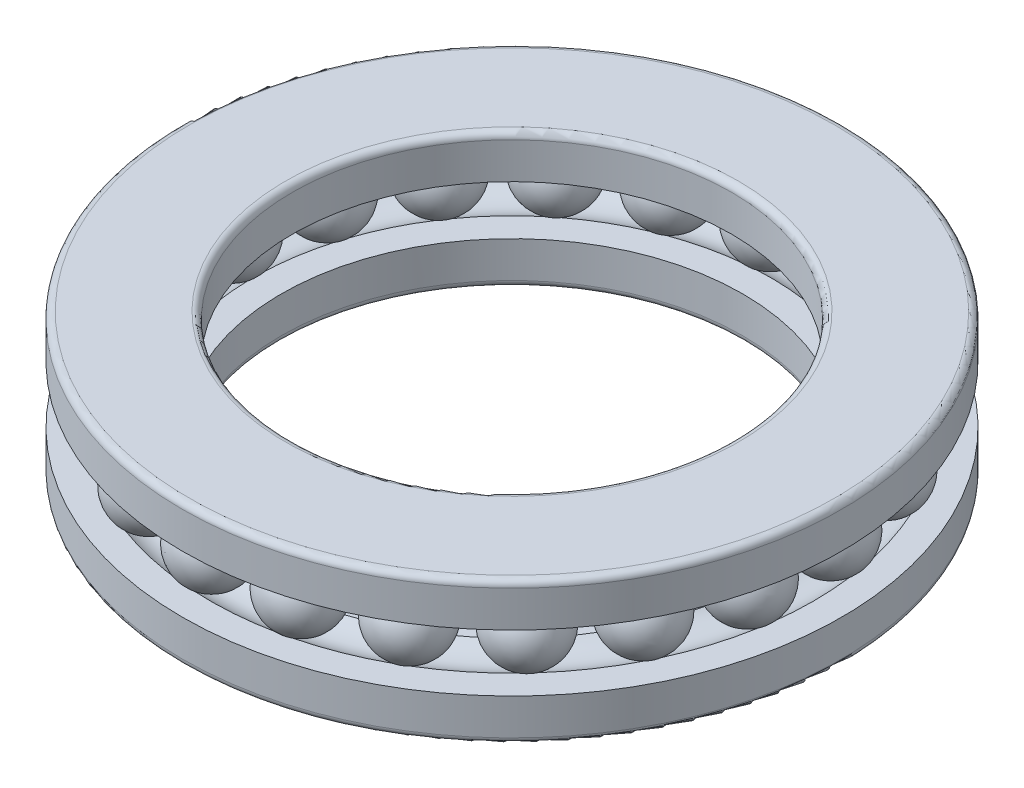
SolidWorks part; units mm, degrees
material "GCr4"
ref_plane "Plane1" through (0, 0, 0) normal (0, 0, 1) x (1, 0, 0)
ref_plane "Plane2" through (0, 0, 0) normal (0, 1, 0) x (1, 0, 0)
ref_plane "Plane3" through (0, 0, 0) normal (1, 0, 0) x (0, 0, -1)
sketch "Dimension Sketch" plane through (0, 0, 0) normal (0, 0, 1) x (1, 0, 0)
  line L0 (0, 0) -> (60, 0)
  point P3 (40, 0)
  point P4 (42, 0)
  point P5 (60, 0)
  point P6 (13, 0)
  point P7 (0.6, 0)
sketch "Sketch1" plane through (0, 0, 0) normal (0, 0, 1) x (1, 0, 0)
  line L0 (30, 0) -> (30, 34.489) construction
  line L1 (0, 0) -> (60, 0)
  line L2 (0, 0) -> (0, 13)
  line L3 (0, 13) -> (60, 13)
  line L4 (60, 0) -> (60, 13)
  line L5 (10, 0) -> (10, 58.489)
  line L6 (50, 0) -> (50, 58.489)
  line L7 (0, 0) -> (0, 58.489)
  line L8 (60, 0) -> (60, 58.489)
  line L9 (9, 0) -> (9, 58.489)
  line L10 (51, 0) -> (51, 58.489)
  line L11 (0, 6.5) -> (60, 6.5) construction
  line L12 (55.5, 0) -> (55.5, 58.489)
  line L13 (4.5, 0) -> (4.5, 58.489)
  line L14 (0, 3.9) -> (250, 3.9)
  line L15 (0, 9.1) -> (250, 9.1)
  circle A0 centre (4.5, 6.5) radius 3.25
sketch "Sketch2" plane through (0, 0, 0) normal (0, 0, 1) x (1, 0, 0)
  line L0 (0, 3.9) -> (250, 3.9) construction
  line L1 (30, 0) -> (30, 34.489) construction
  line L2 (9, 0) -> (9, 58.489) construction
  line L3 (0, 3.9) -> (2.55, 3.9)
  line L4 (0, 0) -> (60, 0)
  line L5 (60, 0) -> (60, 13)
  line L6 (60, 13) -> (0, 13)
  line L7 (0, 13) -> (0, 0)
  line L8 (0, 0) -> (9, 0)
  line L9 (6.45, 3.9) -> (9, 3.9)
  line L11 (0, 3.9) -> (0, 0)
  line L12 (30, 0) -> (30, 34.489) construction
  line L13 (9, 0) -> (9, 3.9)
  circle A0 centre (4.5, 6.5) radius 3.25 construction
  arc A1 (2.55, 3.9) -> (6.45, 3.9) centre (4.5, 6.5) ccw
  dimension "D1" = 0
revolve "Base-Revolve" add sketch "Sketch2" angle 360 about L12
sketch "Sketch3" plane through (0, 0, 0) normal (0, 0, 1) x (1, 0, 0)
  line L2 (4.5, 0) -> (4.5, 58.489) construction
  line L3 (4.5, 0) -> (4.5, 58.489) construction
  line L4 (4.5, 3.2) -> (4.5, 9.8)
  circle A0 centre (4.5, 6.5) radius 3.25 construction
  arc A1 (4.5, 9.75) -> (4.5, 3.25) centre (4.5, 6.5) ccw construction
  arc A2 (4.5, 9.8) -> (4.5, 3.2) centre (4.5, 6.5) ccw
  dimension "D1" = 0.05
revolve "Boss-Revolve2" add sketch "Sketch3" angle 360 about L3
sketch "Sketch4" plane through (0, 0, 0) normal (0, 0, 1) x (1, 0, 0)
  line L0 (30, 0) -> (30, 34.489) construction
  line L1 (0, 9.1) -> (250, 9.1) construction
  line L2 (10, 0) -> (10, 58.489) construction
  line L3 (0, 0) -> (0, 58.489) construction
  line L4 (0, 13) -> (60, 13) construction
  line L5 (30, 0) -> (30, 34.489) construction
  line L6 (0, 9.1) -> (2.55, 9.1)
  line L7 (10, 9.1) -> (10, 13)
  line L8 (0, 9.1) -> (0, 13)
  line L9 (0, 13) -> (10, 13)
  line L12 (6.45, 9.1) -> (10, 9.1)
  circle A0 centre (4.5, 6.5) radius 3.25 construction
  arc A1 (6.45, 9.1) -> (2.55, 9.1) centre (4.5, 6.5) ccw
revolve "Boss-Revolve3" add sketch "Sketch4" angle 360 about L5
pattern_circular "CirPattern1" count 21 over 360 about axis through (30, 0, 0) along (0, 1, 0) of "Boss-Revolve2"
fillet "Fillet1" radius 0.6 4 edges at (30, 13, -20) (30, 13, -30) (30, 0, -21) (30, 0, -30)
equation "\"D1@Sketch1\" = \"DD@Dimension Sketch\""
equation "\"D5@Sketch1\" = \"d1@Dimension Sketch\""
equation "\"D4@Sketch1\" = \"d@Dimension Sketch\""
equation "\"D3@Sketch1\" = \"DD1@Dimension Sketch\""
equation "\"D2@Sketch1\" = \"T@Dimension Sketch\""
equation "\"D1@Fillet1\" = \"r@Dimension Sketch\""
equation "\"D6@Sketch1\" =  ( \"D5@Sketch1\" + \"D1@Sketch1\" )  / 2"
equation "\"D7@Sketch1\" = \"D2@Sketch1\" * 0.4"
equation "\"D8@Sketch1\" = \"D2@Sketch1\" / 2"
equation "\"D1@CirPattern1\" = 3.14*(\"D1@Sketch1\" + \"D5@Sketch1\" )  / 2 / \"D8@Sketch1\"*0.85"
